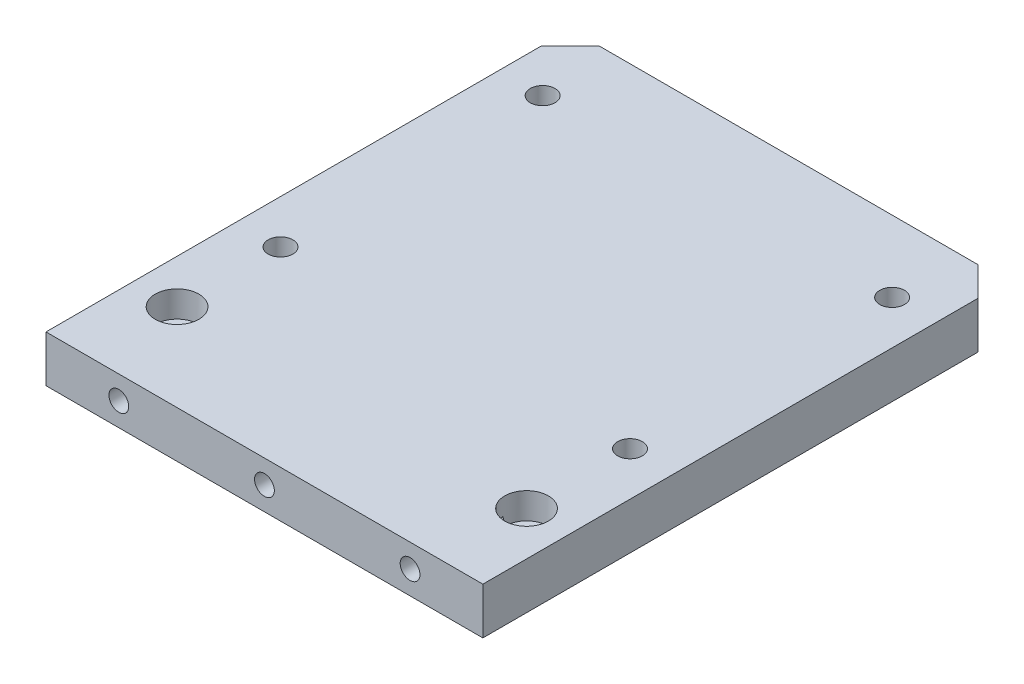
SolidWorks part; units mm, degrees
ref_plane "前视基准面" through (0, 0, 0) normal (0, 0, 1) x (1, 0, 0)
ref_plane "上视基准面" through (0, 0, 0) normal (0, 1, 0) x (1, 0, 0)
ref_plane "右视基准面" through (0, 0, 0) normal (1, 0, 0) x (0, 0, -1)
sketch "草图1" plane through (0, 0, 0) normal (0, 1, 0) x (1, 0, 0)
  line L1 (-75, 90) -> (75, 90)
  line L2 (-75, 90) -> (-75, -90)
  line L3 (-75, -90) -> (75, -90)
  line L4 (75, 90) -> (75, -90)
  line L5 (-75, 90) -> (75, -90) construction
  line L6 (-75, -90) -> (75, 90) construction
  point P0 (0, 0)
  dimension "D1" = 150
  dimension "D2" = 180
extrude "凸台-拉伸1" add sketch "草图1" along normal blind 16
hole_wizard "M8 螺纹孔1" positions "草图2" profile "草图3" tap size "M8" standard "GB"
sketch "草图2" plane through (0, 0, 90) normal (0, 0, 1) x (1, 0, 0)
  line L0 (0, 0) -> (0, 36.5167) construction
  line L2 (-75, 8) -> (-33.5072, 8) construction
  line L3 (-75, 16) -> (-75, 0) construction
  point P0 (-50, 8)
  point P2 (0, 8)
  point P4 (50, 8)
  dimension "D1" = 100
sketch "草图3" plane through (-50, 8, 90) normal (1, 0, 0) x (0, -1, 0)
  line L0 (0, 0) -> (0, 31.2929)
  line L1 (0, 31.2929) -> (3.4, 29.25)
  line L2 (3.4, 29.25) -> (3.4, 0)
  line L5 (3.4, 0) -> (0, 0)
  line L10 (0, 31.2929) -> (-3.4, 29.25) construction
  line L11 (0, -6.35) -> (0, 107.95) construction
  dimension "螺纹孔钻头直径" = 6.8
  dimension "螺纹孔钻头深度" = 29.25
  dimension "导头角度" = 118
cosmetic thread "孔螺蚊线1" parameters "D1"=16, "D2"=8
cosmetic thread "孔螺蚊线2" parameters "D1"=16, "D2"=8
cosmetic thread "孔螺蚊线3" parameters "D1"=16, "D2"=8
hole_wizard "打孔尺寸(%根据)内六角圆柱头螺钉的类型1" positions "草图4" profile "草图5" counterbore size "M8" standard "GB"
sketch "草图4" plane through (0, 16, 0) normal (0, 1, 0) x (1, 0, 0)
  line L0 (0, 0) -> (0, 38.0849) construction
  line L2 (-75, 90) -> (-75, -90) construction
  line L3 (-75, -90) -> (75, -90) construction
  point P0 (-60, -60)
  point P2 (60, -60)
  dimension "D1" = 15
  dimension "D2" = 30
sketch "草图5" plane through (-60, 16, 60) normal (1, 0, 0) x (0, 0, 1)
  line L0 (0, 0) -> (0, 31.9539)
  line L1 (0, 31.9539) -> (4.5, 29.25)
  line L2 (4.5, 29.25) -> (4.5, 9)
  line L3 (4.5, 9) -> (7.5, 9)
  line L4 (7.5, 9) -> (7.5, 0)
  line L5 (7.5, 0) -> (0, 0)
  line L10 (0, 31.9539) -> (-4.5, 29.25) construction
  line L11 (0, -6.35) -> (0, 107.95) construction
  dimension "孔直径" = 9
  dimension "孔深度" = 29.25
  dimension "柱形沉头孔直径" = 15
  dimension "柱形沉头孔深度" = 9
  dimension "导头角度" = 118
hole_wizard "M10 螺纹孔1" positions "草图6" profile "草图7" tap size "M10" standard "GB" end condition through all
sketch "草图6" plane through (0, 16, 0) normal (0, 1, 0) x (1, 0, 0)
  line L0 (0, 0) -> (0, 70.7271) construction
  line L2 (75, 90) -> (-75, 90) construction
  point P0 (-60, 65.5198)
  point P2 (60, 65.5198)
  point P4 (-60, -24.4802)
  point P6 (60, -24.4802)
  dimension "D1" = 24.4802
  dimension "D2" = 90
  dimension "D3" = 120
sketch "草图7" plane through (-60, 16, -65.5198) normal (1, 0, 0) x (0, 0, 1)
  line L0 (0, 0) -> (0, 16)
  line L1 (0, 16) -> (4.25, 16)
  line L2 (4.25, 16) -> (4.25, 0)
  line L5 (4.25, 0) -> (0, 0)
  line L11 (0, -6.35) -> (0, 107.95) construction
  dimension "通孔螺纹孔钻头直径" = 8.5
  dimension "通孔螺纹孔钻头深度" = 16
cosmetic thread "孔螺蚊线4" parameters "D2"=10
cosmetic thread "孔螺蚊线5" parameters "D2"=10
cosmetic thread "孔螺蚊线6" parameters "D2"=10
cosmetic thread "孔螺蚊线7" parameters "D2"=10
chamfer "倒角1" distance 10 angle 45 2 edges at (-75, 8, -90) (75, 8, -90)
